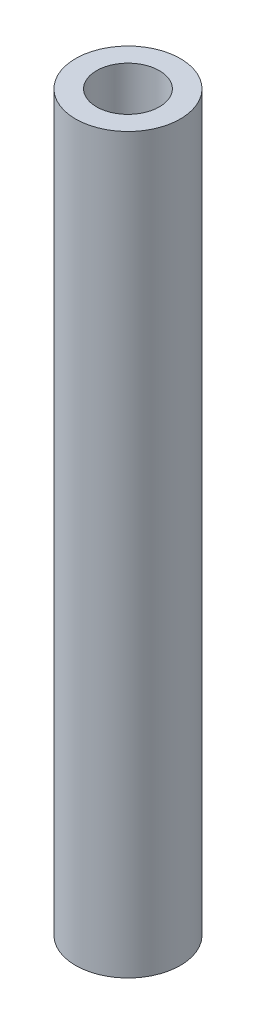
from build123d import *

# Parameters (mm, degrees)
SKETCH1_R           = 2.5
SKETCH1_R_2         = 1.5
BOSS_EXTRUDE1_DEPTH = 35
SKETCH2_R           = 1.5
SKETCH2_R_2         = 0.5
BOSS_EXTRUDE2_DEPTH = 2


with BuildPart() as part:
    # Sketch1 → Boss-Extrude1 (new body)
    with BuildSketch(Plane(origin=(0, 0, 0), x_dir=(1, 0, 0), z_dir=(0, 1, 0))):
        with Locations(Location((0, 0, 0), (0, 0, 270))):
            Circle(SKETCH1_R)
        with Locations(Location((0, 0, 0), (0, 0, 270))):
            Circle(SKETCH1_R_2, mode=Mode.SUBTRACT)
    extrude(amount=BOSS_EXTRUDE1_DEPTH)

    # Sketch2 → Boss-Extrude2 (add)
    with BuildSketch(Plane.XZ):
        with Locations(Location((0, 0, 0), (0, 0, 270))):
            Circle(SKETCH2_R)
        with Locations(Location((0, 0, 0), (0, 0, 270))):
            Circle(SKETCH2_R_2, mode=Mode.SUBTRACT)
    extrude(amount=-BOSS_EXTRUDE2_DEPTH)


solid = part.part
